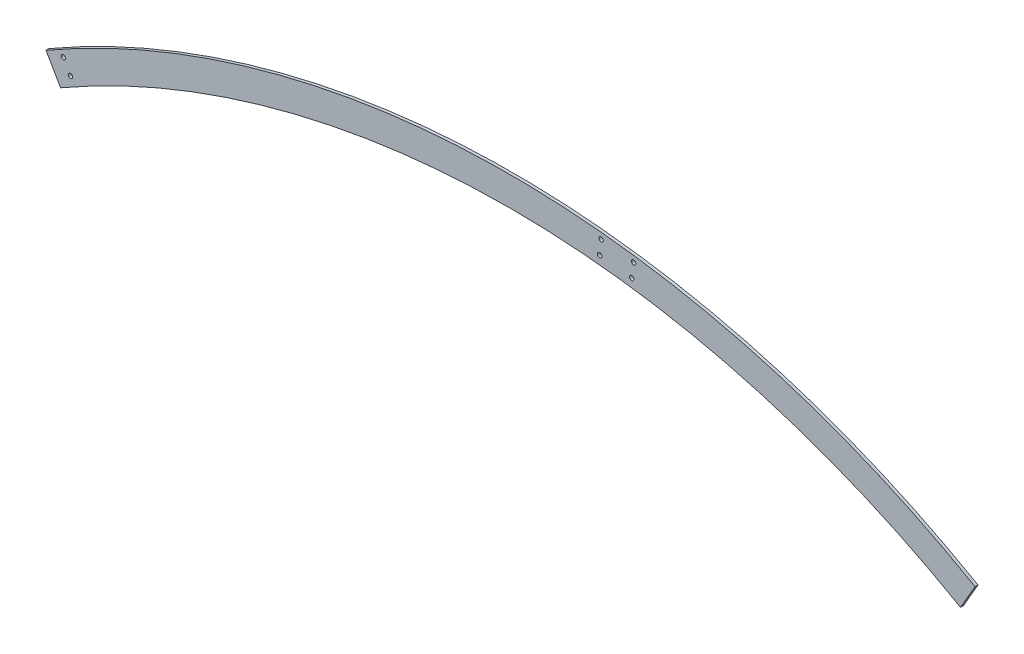
from build123d import *

# Parameters (mm, degrees)
BOSS_EXTRUDE1_DEPTH        = 8
F_12_0_12_DIAMETER_HOLE1_D = 12


with BuildPart() as part:
    # Sketch1 → Boss-Extrude1 (new body)
    with BuildSketch(Plane.XY):
        with BuildLine():
            Line((-1275, 69.282032303), (-1235, 0))
            ThreePointArc((-1235, 0), (0, 330.917252652), (1235, 0))
            Line((1235, 0), (1275, 69.282032303))
            ThreePointArc((1275, 69.282032303), (0, 410.917252652), (-1275, 69.282032303))
        make_face()
    extrude(amount=BOSS_EXTRUDE1_DEPTH)

    # Ø12.0 (12) Diameter Hole1 (through all)
    with Locations(Plane.XY.offset(8)):
        with Locations((-1227.328979234, 76.713402287), (-1207.947550426, 41.722543232), (248.497397062, 381.698489423), (244.573237614, 341.891442652), (337.892259182, 371.279342309), (332.556416163, 331.636830036)):
            Hole(F_12_0_12_DIAMETER_HOLE1_D / 2)


solid = part.part
